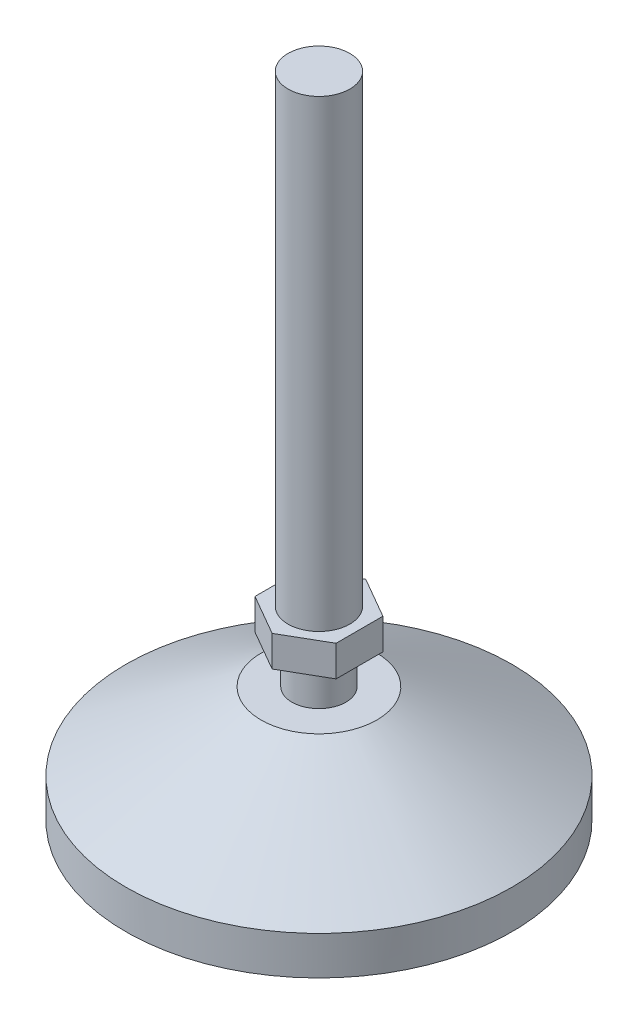
from build123d import *

# Parameters (mm, degrees)
SKETCH_2_R      = 7
EXTRUDE_1_DEPTH = 10
EXTRUDE_2_DEPTH = 8
SKETCH_4_R      = 8
EXTRUDE_3_DEPTH = 120


with BuildPart() as part:
    # 草图1 → 旋转1 (revolve)
    with BuildSketch(Plane.XY, mode=Mode.PRIVATE) as revolve_1_sk:
        Polygon((0, 30), (0, 0), (50, 0), (50, 10), (15, 30), align=None)
    revolve(revolve_1_sk.sketch.rotate(Axis((0, 30, 0), (0, -1, 0)), 180), axis=Axis((0, 30, 0), (0, -1, 0)))

    # 草图2 → 凸台-拉伸1 (add)
    with BuildSketch(Plane(origin=(0, 30, 0), x_dir=(1, 0, 0), z_dir=(0, 1, 0))):
        Circle(SKETCH_2_R)
    extrude(amount=EXTRUDE_1_DEPTH)

    # 草图3 → 凸台-拉伸2 (add)
    with BuildSketch(Plane(origin=(0, 40, 0), x_dir=(1, 0, 0), z_dir=(0, 1, 0))):
        Polygon((0, 12.124355653), (-10.5, 6.062177826), (-10.5, -6.062177826), (0, -12.124355653), (10.5, -6.062177826), (10.5, 6.062177826), align=None)
    extrude(amount=EXTRUDE_2_DEPTH)

    # 草图4 → 凸台-拉伸3 (add)
    with BuildSketch(Plane(origin=(0, 48, 0), x_dir=(1, 0, 0), z_dir=(0, 1, 0))):
        with Locations(Location((0, 0, 0), (0, 0, 270))):
            Circle(SKETCH_4_R)
    extrude(amount=EXTRUDE_3_DEPTH)


solid = part.part
